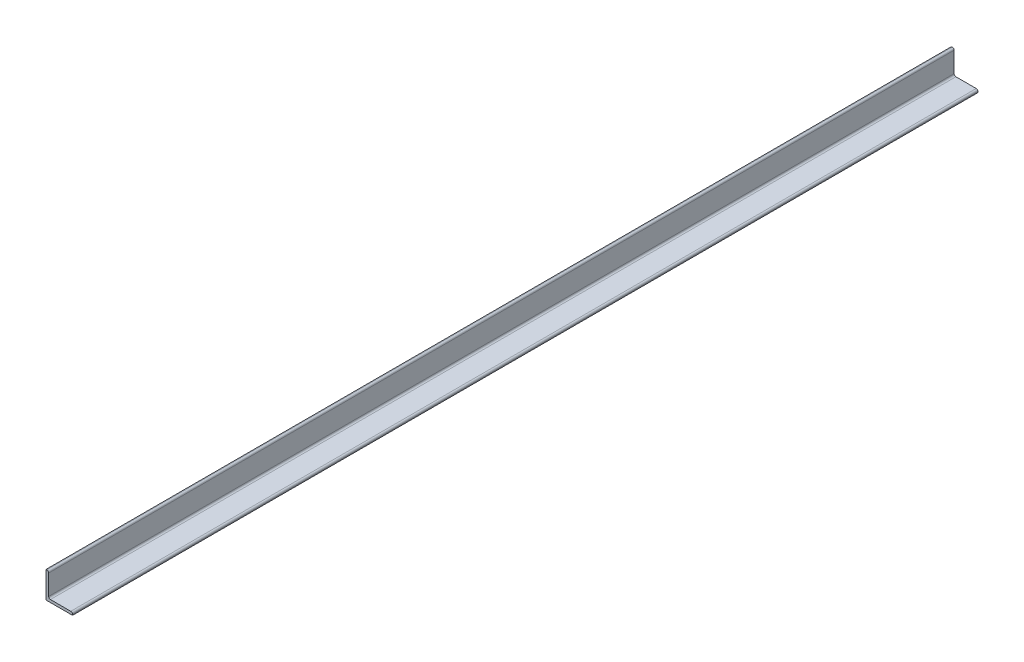
from build123d import *

# Parameters (mm, degrees)
BOSS_EXTRUDE1_DEPTH = 1024


with BuildPart() as part:
    # Sketch1 → Boss-Extrude1 (new body)
    with BuildSketch(Plane.XY):
        with BuildLine():
            Line((0, 0), (30, 0))
            Line((30, 0), (30, 1))
            ThreePointArc((30, 1), (29.414213562, 2.414213562), (28, 3))
            Line((28, 3), (5, 3))
            ThreePointArc((5, 3), (3.585786438, 3.585786438), (3, 5))
            Line((3, 5), (3, 28))
            ThreePointArc((3, 28), (2.414213562, 29.414213562), (1, 30))
            Line((1, 30), (0, 30))
            Line((0, 30), (0, 0))
        make_face()
    extrude(amount=BOSS_EXTRUDE1_DEPTH)


solid = part.part
